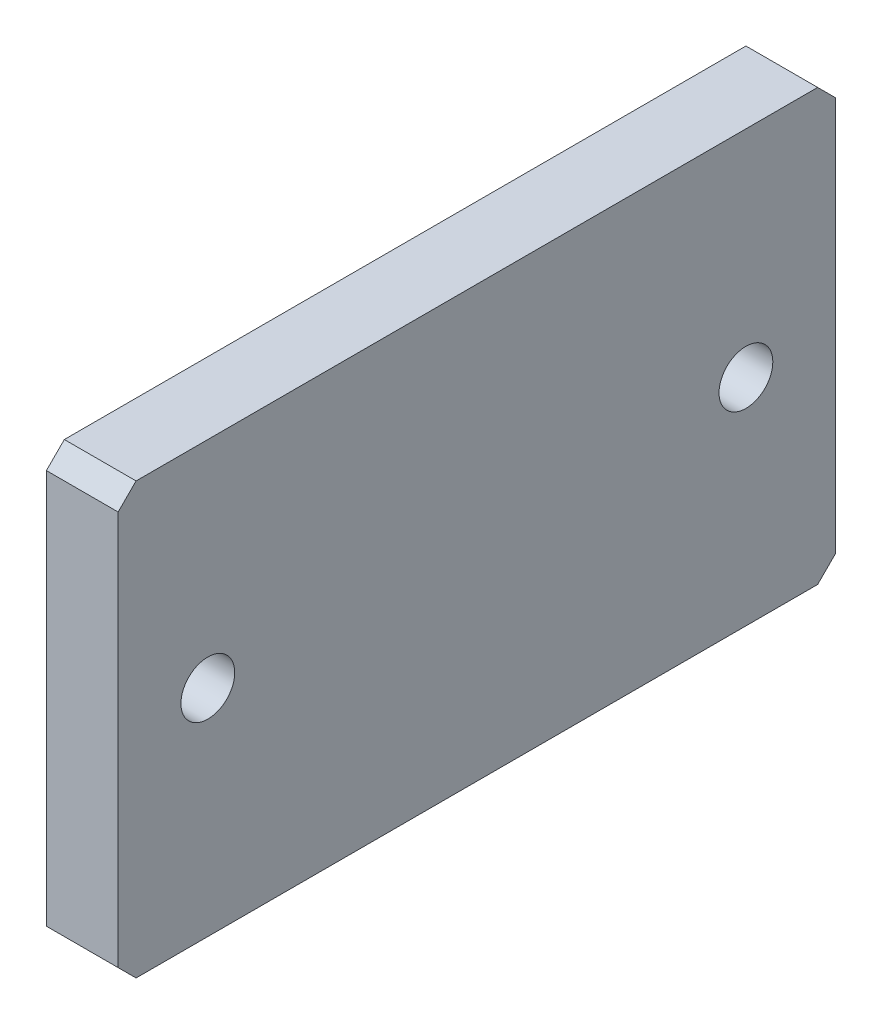
from build123d import *

# Parameters (mm, degrees)
SKETCH_1_W              = 200
SKETCH_1_H              = 120
EXTRUDE_1_DEPTH         = 20
HOLE_WIZARD_15_0_15_1_D = 15
CHAMFER_1_SIZE          = 5


with BuildPart() as part:
    # 草图1 → 凸台-拉伸1 (new body)
    with BuildSketch(Plane(origin=(0, 0, 0), x_dir=(0, 0, -1), z_dir=(1, 0, 0))):
        Rectangle(SKETCH_1_W, SKETCH_1_H)
    extrude(amount=EXTRUDE_1_DEPTH)

    # Ø15.0 (15) 直径孔1 (through all)
    with Locations(Plane(origin=(20, 0, 0), x_dir=(0, 0, -1), z_dir=(1, 0, 0))):
        with Locations((-75, 0), (75, 0)):
            Hole(HOLE_WIZARD_15_0_15_1_D / 2)

    # 倒角1
    chamfer_1_edges = [part.edges().sort_by_distance(p)[0] for p in [
        (10, -60, -100),
        (10, -60, 100),
        (10, 60, 100),
        (10, 60, -100),
    ]]
    chamfer(chamfer_1_edges, length=CHAMFER_1_SIZE)


solid = part.part
